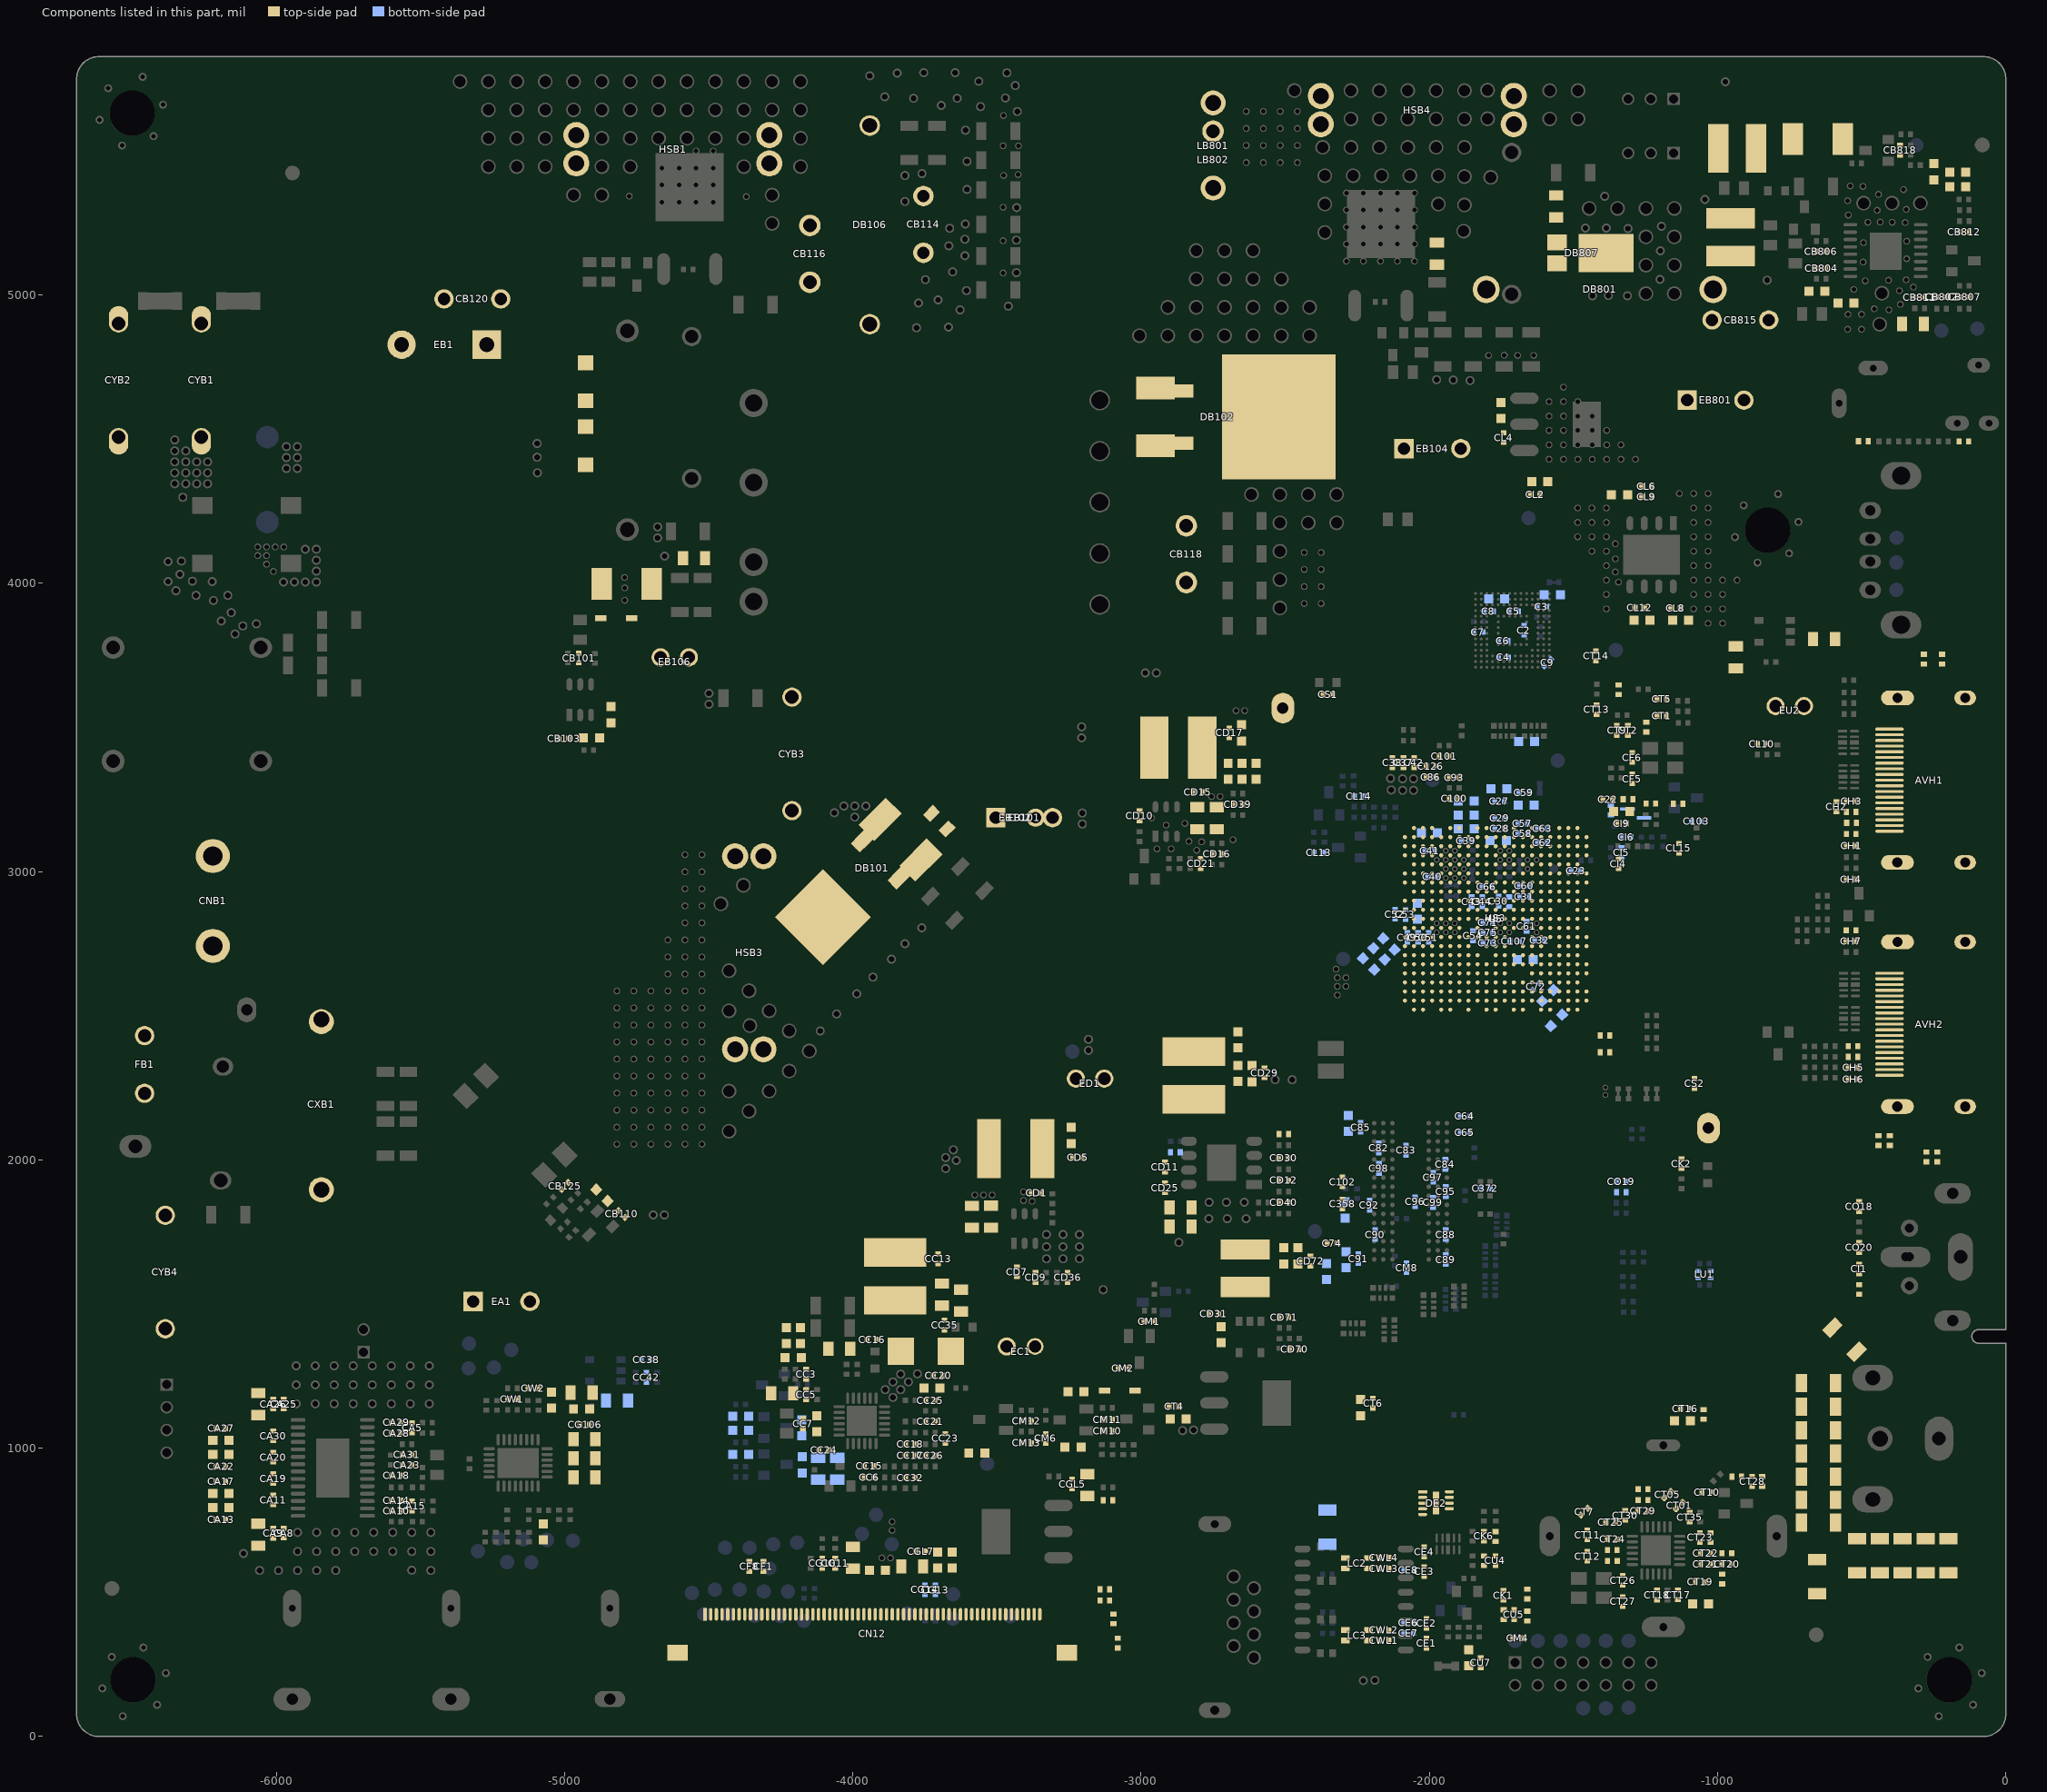
[diagram p0: the components of this part, seen from the top]
# Altium PCB MISC84395.PcbDoc (part 5 of 26)
Units mil, origin at the board's own origin, x right, y up, seen from the top; angles counter-clockwise.
Board outline 6692.91 x 5826.77 mil, 2 copper layers (TopLayer, BottomLayer), stack 61.855 mil thick; 951 components, 565 nets, 4374 pads, 1804 vias.
Unrouted connection lines stored in the file: 1.

## Footprints (in the part's own frame and the unit in brackets; to place one, negate y for a bottom-side part, rotate by r counter-clockwise, add the part's x,y. Pads: shape width x height; smd on the part's side, far side on the other; paste and mask are expansions set on the pad) (continued)
BGA406/0.8 [mm] "Mstar,MSD6A648WT-003J,16.12.17"
  round 0.36 smd: A2(-7.2,8) A3(-6.4,8) A5(-4.8,8) A6(-4,8) A8(-2.4,8) A9(-1.6,8) A11(0,8) A12(0.8,8) A14(2.4,8) A16(4,8) A17(4.8,8) A19(6.4,8) A20(7.2,8) AA2(-7.2,-8) AA3(-6.4,-8) AA4(-5.6,-8) AA6(-4,-8) AA7(-3.2,-8) AA9(-1.6,-8) AA10(-0.8,-8) AA12(0.8,-8) AA13(1.6,-8) AA15(3.2,-8) AA16(4,-8) AA18(5.6,-8) AA19(6.4,-8) AA20(7.2,-8) B1(-8,7.2) B2(-7.2,7.2) B3(-6.4,7.2) B4(-5.6,7.2) B5(-4.8,7.2) B6(-4,7.2) B7(-3.2,7.2) B8(-2.4,7.2) B9(-1.6,7.2) B10(-0.8,7.2) B11(0,7.2) B12(0.8,7.2) B13(1.6,7.2) B14(2.4,7.2) B15(3.2,7.2) B16(4,7.2) B17(4.8,7.2) B18(5.6,7.2) B19(6.4,7.2) B20(7.2,7.2) C1(-8,6.4) C2(-7.2,6.4) C3(-6.4,6.4) C4(-5.6,6.4) C5(-4.8,6.4) C6(-4,6.4) C7(-3.2,6.4) C8(-2.4,6.4) C9(-1.6,6.4) C10(-0.8,6.4) C11(0,6.4) C12(0.8,6.4) C13(1.6,6.4) C14(2.4,6.4) C15(3.2,6.4) C16(4,6.4) C17(4.8,6.4) C18(5.6,6.4) C19(6.4,6.4) C20(7.2,6.4) C21(8,6.4) D2(-7.2,5.6) D3(-6.4,5.6) D4(-5.6,5.6) D5(-4.8,5.6) D6(-4,5.6) D7(-3.2,5.6) D8(-2.4,5.6) D9(-1.6,5.6) D10(-0.8,5.6) D11(0,5.6) D12(0.8,5.6) D13(1.6,5.6) D14(2.4,5.6) D15(3.2,5.6) D16(4,5.6) D17(4.8,5.6) D18(5.6,5.6) D19(6.4,5.6) D20(7.2,5.6) D21(8,5.6) E1(-8,4.8) E2(-7.2,4.8) E3(-6.4,4.8) E4(-5.6,4.8) E5(-4.8,4.8) E6(-4,4.8) E7(-3.2,4.8) E10(-0.8,4.8) E11(0,4.8) E12(0.8,4.8) E13(1.6,4.8) E14(2.4,4.8) E15(3.2,4.8) E16(4,4.8) E17(4.8,4.8) E18(5.6,4.8) E19(6.4,4.8) E20(7.2,4.8) E21(8,4.8) F1(-8,4) F2(-7.2,4) F3(-6.4,4) F4(-5.6,4) F5(-4.8,4) F6(-4,4) F7(-3.2,4) F8(-2.4,4) F9(-1.6,4) F10(-0.8,4) F11(0,4) F12(0.8,4) F13(1.6,4) F14(2.4,4) F15(3.2,4) F16(4,4) F17(4.8,4) F18(5.6,4) F19(6.4,4) F20(7.2,4) F21(8,4) G2(-7.2,3.2) G3(-6.4,3.2) G4(-5.6,3.2) G5(-4.8,3.2) G6(-4,3.2) G7(-3.2,3.2) G8(-2.4,3.2) G9(-1.6,3.2) G10(-0.8,3.2) G11(0,3.2) G13(1.6,3.2) G14(2.4,3.2) G15(3.2,3.2) G16(4,3.2) G17(4.8,3.2) G18(5.6,3.2) G19(6.4,3.2) G20(7.2,3.2) G21(8,3.2) H1(-8,2.4) H2(-7.2,2.4) H3(-6.4,2.4) H4(-5.6,2.4) H6(-4,2.4) H7(-3.2,2.4) H8(-2.4,2.4) H10(-0.8,2.4) H11(0,2.4) H12(0.8,2.4) H14(2.4,2.4) H15(3.2,2.4) H16(4,2.4) H17(4.8,2.4) H18(5.6,2.4) H19(6.4,2.4) H20(7.2,2.4) H21(8,2.4) J1(-8,1.6) J2(-7.2,1.6) J3(-6.4,1.6) J4(-5.6,1.6) J5(-4.8,1.6) J6(-4,1.6) J7(-3.2,1.6) J10(-0.8,1.6) J11(0,1.6) J12(0.8,1.6) J13(1.6,1.6) J14(2.4,1.6) J15(3.2,1.6) J16(4,1.6) J17(4.8,1.6) J18(5.6,1.6) J19(6.4,1.6) J20(7.2,1.6) J21(8,1.6) K2(-7.2,0.8) K3(-6.4,0.8) K4(-5.6,0.8) K5(-4.8,0.8) K6(-4,0.8) K7(-3.2,0.8) K8(-2.4,0.8) K9(-1.6,0.8) K10(-0.8,0.8) K11(0,0.8) K13(1.6,0.8) K15(3.2,0.8) K16(4,0.8) K17(4.8,0.8) K18(5.6,0.8) K19(6.4,0.8) K20(7.2,0.8) K21(8,0.8) L1(-8,0) L2(-7.2,0) L3(-6.4,0) L4(-5.6,0) L5(-4.8,0) L6(-4,0) L7(-3.2,0) L8(-2.4,0) L9(-1.6,0) L10(-0.8,0) L11(0,0) L12(0.8,0) L13(1.6,0) L14(2.4,0) L15(3.2,0) L16(4,0) L17(4.8,0) L18(5.6,0) L19(6.4,0) L20(7.2,0) M1(-8,-0.8) M2(-7.2,-0.8) M5(-4.8,-0.8) M6(-4,-0.8) M7(-3.2,-0.8) M8(-2.4,-0.8) M9(-1.6,-0.8) M10(-0.8,-0.8) M11(0,-0.8) M12(0.8,-0.8) M13(1.6,-0.8) M14(2.4,-0.8) M15(3.2,-0.8) M16(4,-0.8) M17(4.8,-0.8) M18(5.6,-0.8) M19(6.4,-0.8) M20(7.2,-0.8) M21(8,-0.8) N1(-8,-1.6) N2(-7.2,-1.6) N3(-6.4,-1.6) N4(-5.6,-1.6) N5(-4.8,-1.6) N6(-4,-1.6) N7(-3.2,-1.6) N8(-2.4,-1.6) N9(-1.6,-1.6) N10(-0.8,-1.6) N11(0,-1.6) N12(0.8,-1.6) N13(1.6,-1.6) N14(2.4,-1.6) N15(3.2,-1.6) N16(4,-1.6) N17(4.8,-1.6) N18(5.6,-1.6) N19(6.4,-1.6) N20(7.2,-1.6) N21(8,-1.6) P2(-7.2,-2.4) P3(-6.4,-2.4) P4(-5.6,-2.4) P5(-4.8,-2.4) P6(-4,-2.4) P7(-3.2,-2.4) P8(-2.4,-2.4) P9(-1.6,-2.4) P10(-0.8,-2.4) P11(0,-2.4) P12(0.8,-2.4) P13(1.6,-2.4) P14(2.4,-2.4) P15(3.2,-2.4) P16(4,-2.4) P17(4.8,-2.4) P18(5.6,-2.4) P19(6.4,-2.4) P20(7.2,-2.4) R1(-8,-3.2) R2(-7.2,-3.2) R3(-6.4,-3.2) R4(-5.6,-3.2) R5(-4.8,-3.2) R6(-4,-3.2) R7(-3.2,-3.2) R8(-2.4,-3.2) R9(-1.6,-3.2) R10(-0.8,-3.2) R11(0,-3.2) R12(0.8,-3.2) R13(1.6,-3.2) R14(2.4,-3.2) R15(3.2,-3.2) R16(4,-3.2) R17(4.8,-3.2) R18(5.6,-3.2) R19(6.4,-3.2) R20(7.2,-3.2) R21(8,-3.2) T1(-8,-4) T2(-7.2,-4) T3(-6.4,-4) T4(-5.6,-4) T5(-4.8,-4) T6(-4,-4) T7(-3.2,-4) T8(-2.4,-4) T9(-1.6,-4) T10(-0.8,-4) T11(0,-4) T12(0.8,-4) T13(1.6,-4) T14(2.4,-4) T15(3.2,-4) T16(4,-4) T17(4.8,-4) T18(5.6,-4) T19(6.4,-4) T20(7.2,-4) T21(8,-4) U2(-7.2,-4.8) U3(-6.4,-4.8) U4(-5.6,-4.8) U5(-4.8,-4.8) U6(-4,-4.8) U7(-3.2,-4.8) U8(-2.4,-4.8) U9(-1.6,-4.8) U10(-0.8,-4.8) U11(0,-4.8) U12(0.8,-4.8) U13(1.6,-4.8) U14(2.4,-4.8) U15(3.2,-4.8) U16(4,-4.8) U17(4.8,-4.8) U18(5.6,-4.8) U19(6.4,-4.8) U20(7.2,-4.8) V1(-8,-5.6) V2(-7.2,-5.6) V3(-6.4,-5.6) V4(-5.6,-5.6) V5(-4.8,-5.6) V6(-4,-5.6) V7(-3.2,-5.6) V8(-2.4,-5.6) V9(-1.6,-5.6) V10(-0.8,-5.6) V11(0,-5.6) V12(0.8,-5.6) V13(1.6,-5.6) V14(2.4,-5.6) V15(3.2,-5.6) V16(4,-5.6) V17(4.8,-5.6) V18(5.6,-5.6) V19(6.4,-5.6) V20(7.2,-5.6) V21(8,-5.6) W1(-8,-6.4) W2(-7.2,-6.4) W3(-6.4,-6.4) W4(-5.6,-6.4) W5(-4.8,-6.4) W6(-4,-6.4) W7(-3.2,-6.4) W8(-2.4,-6.4) W9(-1.6,-6.4) W10(-0.8,-6.4) W11(0,-6.4) W12(0.8,-6.4) W13(1.6,-6.4) W14(2.4,-6.4) W15(3.2,-6.4) W16(4,-6.4) W17(4.8,-6.4) W18(5.6,-6.4) W19(6.4,-6.4) W20(7.2,-6.4) W21(8,-6.4) Y1(-8,-7.2) Y2(-7.2,-7.2) Y3(-6.4,-7.2) Y4(-5.6,-7.2) Y5(-4.8,-7.2) Y6(-4,-7.2) Y7(-3.2,-7.2) Y8(-2.4,-7.2) Y9(-1.6,-7.2) Y10(-0.8,-7.2) Y11(0,-7.2) Y12(0.8,-7.2) Y13(1.6,-7.2) Y14(2.4,-7.2) Y15(3.2,-7.2) Y16(4,-7.2) Y17(4.8,-7.2) Y18(5.6,-7.2) Y19(6.4,-7.2) Y20(7.2,-7.2) Y21(8,-7.2)
  round 0.36 smd mask+0.102: B21(8,7.2)
  silkscreen extent -9.62,-8.8 8.8,9.67, body extent -8.8,-8.8 8.8,8.8, height 1.6
C0402#1 [mm] "片式电容  2018.10.7 替换为兼容0201封装"
  rect 0.45x0.5 smd mask+0.051: 1(-0.425,0) 1(-0.425,0) 2(0.425,0) 2(0.425,0)
  silkscreen extent -0.88,-0.4 0.88,0.4
C0402#2 [mm] "片式电容  2018.10.7 替换为兼容0201封装"
  rrect50% 0.45x0.5 smd mask+0.051: 1(-0.425,0) 2(0.425,0)
  rect 0.3x0.3 smd mask+0.051: 1(-0.25,0) 2(0.25,0)
  rect 0.6x0.6 on Top Solder: 2(0,0)
  TopLayer pour cut-out: -0.318,0.302 -0.318,-0.303 0.306,-0.303 0.306,0.302
  silkscreen extent -0.88,-0.4 0.88,0.4, body extent -0.5,-0.25 0.5,0.25, height 0.5
C0603 [mm] "片式电容"
  rect 0.8x0.8 smd mask+0.076: 1(-0.706,0) 2(0.706,0)
  silkscreen extent -1.39,-0.55 1.39,0.55, body extent -0.8,-0.4 0.8,0.4, height 0.8
C0805 [mm] "片式电容"
  rect 0.9x1.25 smd mask+0.076: 1(-0.966,0) 2(0.966,0)
  silkscreen extent -1.73,-0.78 1.73,0.78, body extent -1,-0.62 1,0.63, height 1.25
C1206 [mm] "片式电容"
  rect 1x1.6 smd mask+0.076: 1(-1.5,-0.001) 2(1.5,0.001)
  silkscreen extent -2.39,-0.95 2.39,0.95, body extent -1.6,-0.8 1.6,0.8, height 1.3
CAP6.5*5-V-5-1 [mm] "TDK，CC45SL3DD680JYSNA，外K型引脚，AI，0713_2018"
  round 2.1 on Top Overlay: 0(-2.5,0) 0(2.5,0)
  round 1.9 hole 1.2 mask+0.051: 1(-2.5,0) 2(2.5,0)
  BottomLayer lines w0.6: -2.19,0.39 -4.056,1.556 ; 2.89,0.31 4.056,-1.556 ; -2.5,0 -4.056,1.556 ; 2.5,0 4.056,-1.556 ; -2.89,-0.31 -4.056,1.556 ; 2.19,-0.39 4.056,-1.556
  silkscreen extent -5.5,-2.5 5.5,2.5
CAP7.5*2.5-V-5 [mm] "同皓电子"
  round 1.7 hole 1.1: 1(-2.5,0) 2(2.5,0)
  round 1.9 on Top Overlay: 43(2.5,0) 44(-2.5,0)
  BottomLayer lines w0.6: -2.89,-0.31 -2.92,-0.262 ; -2.5,0 -2.729,0.229 -4.056,1.556 ; -2.19,0.39 -2.238,0.42 ; 2.19,-0.39 2.238,-0.42 2.5,-0.584 4.056,-1.556 ; 2.5,0 4.056,-1.556 ; 2.89,0.31 2.92,0.262 4.056,-1.556 ; -4.056,1.556 -2.238,0.42 ; -4.056,1.556 -3.035,-0.078 -2.92,-0.262 ; -2.92,-0.262 -2.92,-0.262 ; -2.92,-0.262 -2.92,-0.262 ; -2.238,0.42 -2.238,0.42 ; -2.238,0.42 -2.238,0.42
  silkscreen extent -3.75,-1.25 3.75,1.25, body extent -3.75,-1.25 3.75,1.25, height 8.5
CAP8*2.5-V-5 [mm] "C242G472J20A201(编带/法拉)"
  round 1.8 hole 1.1: 1(-2.5,0) 2(2.5,0)
  round 2 on Top Overlay: 1(-2.5,0) 1(2.5,0)
  BottomLayer lines w0.6: 2.15,-0.456 4.056,-1.556 ; -2.956,-0.35 -4.056,1.556 ; 2.5,0 4.056,-1.556 ; -2.5,0 -4.056,1.556 ; 2.956,0.35 3.157,0 4.056,-1.556 ; -2.15,0.456 -4.056,1.556
  silkscreen extent -4,-1.25 4,1.25
CAP8.5*5-V-5 [mm] "TDK，CC45SL3AD221JYSNA，外K型引脚，AI，0713_2018"
  round 2.1 on Top Overlay: 0(-2.5,0) 0(2.5,0)
  round 1.9 hole 1.2 mask+0.051: 1(-2.5,0) 2(2.5,0)
  BottomLayer lines w0.6: 2.19,-0.39 4.056,-1.556 ; -2.89,-0.31 -4.056,1.556 ; 2.5,0 4.056,-1.556 ; -2.5,0 -4.056,1.556 ; 2.89,0.31 4.056,-1.556 ; -2.19,0.39 -4.056,1.556
  silkscreen extent -5.5,-2.5 5.5,2.5
CAP10*4.5-V-5 [mm] "YU102472M090DAND5H，陶瓷电容，17.12.22"
  round 1.7 hole 1.1: 1(-2.5,0) 2(2.5,0)
  round 1.9 on Top Overlay: 41(2.5,0) 42(-2.5,0)
  BottomLayer lines w0.6: -2.89,-0.31 -2.92,-0.262 ; -2.5,0 -4.056,1.556 ; -2.19,0.39 -2.238,0.42 ; 2.19,-0.39 2.238,-0.42 ; 2.5,0 4.056,-1.556 ; 2.89,0.31 2.92,0.262 ; -4.056,1.556 -2.92,-0.262 ; -4.056,1.556 -2.238,0.42 ; -2.92,-0.262 -2.92,-0.262 ; -2.92,-0.262 -2.92,-0.262 ; -2.238,0.42 -2.238,0.42 ; -2.238,0.42 -2.238,0.42 ; 2.238,-0.42 2.238,-0.42 ; 2.238,-0.42 2.238,-0.42 ; 2.238,-0.42 2.439,-0.545 4.056,-1.556 ; 2.92,0.262 2.92,0.262 4.056,-1.556 ; 2.92,0.262 2.92,0.262
  silkscreen extent -5.55,-2.25 5.55,2.25
CAP13*5-V-10-1#1 [mm] "Walsin;YU1AH471M060DAMD0H;160718（18.03.15  更新孔径）"
  oval 2.35x1.7 hole 1.2 copper offset -0.375,0: 1(-5,0)
  oval 2.35x1.7 hole 1.2 copper offset 0.375,0: 2(5,0)
  oval 2.55x1.9 on Top Overlay: 61(-5,0) 61(5,0)
  silkscreen extent -5.71,-3 5.81,3
CAP13*5-V-10-1#2 [mm] "Walsin;YU1AH471M060DAMD0H;160718（18.03.15  更新孔径）"
  round 1.7 hole 1.2: 1(-5,0) 2(5,0)
  round 1.9 on Top Overlay: 61(-5,0) 61(5,0)
  silkscreen extent -5.71,-3 5.81,3
CAP18*8.5-V-15 [mm] "PX334K3ID49H200D9R(凯励)(18.01.12更新孔径）(18.07.18 更新丝印框，加了公差）"
  round 2.2 hole 1.4: 1(-7.5,0)
  round 2.2 hole 1.4 copper offset -0.2,0: 2(7.5,0)
  round 2.4 on Top Overlay: 77(7.5,0) 78(-7.5,0)
  silkscreen extent -9.25,-4.45 9.25,4.45
CAUTION [mil]
  silkscreen extent -400,-146 486,161
COLD [mil]
CON2-H7.92 [mm] "因物料底部露金属，20170630增加1.8mm安规禁布"
  round 3 / inner round 3 / far side round 4.4 hole 1.7: 1(0,3.96) 3(0,-3.96)
  round 3.2 on Top Overlay: 109(0,3.96) 110(0,-3.96)
  silkscreen extent -12,-6.52 4.27,8.46, body extent -11.46,-6.04 0.56,5.86, height 8.49
"Conformal Coating" [mm] "三防漆虚线框"
  round 0.3 on Mech2: 0(0,0)
CQC [mil]
D1-H-17.5 [mm] "FR107 二极管与FR207 共用封装"
  round 2 on Top Overlay: 0(-8.75,0) 1(8.75,0)
  round 1.8 hole 1.3: A(-8.75,0) K(8.75,0)
  BottomLayer lines w0.6: -8.675,0.569 -6.55,0 ; 8.675,0.569 6.55,0 ; -8.75,0 -6.55,0 ; 8.75,0 6.55,0 ; -8.675,-0.569 -6.55,0 ; 8.675,-0.569 6.55,0
  silkscreen extent -7.8,-1.65 7.7,1.65, body extent -9.13,-1.49 9.13,1.5, height 3.15
D2PAK3#1 [mm] "伟达电子；SFS1006G;增加TO-252兼容；160309"
  oval 2.794x1.143 smd: 1(5.542,-2.2) 3(5.542,2.4)
  rect 2.794x1.143 smd: 1(5.544,-2.2) 3(5.544,2.4)
  rect 3.4x2 smd paste-5 mask-5: 1(7.494,-2.44) 3(7.494,2.64)
  rect 6x6 smd paste-10 mask-11: 2(-2.159,0.1)
  TopLayer pour cut-out: 3.373,2.4 6.497,2.4 6.497,-2.245 6.438,-2.54 6.271,-2.791 6.02,-2.958 5.725,-3.017 5.725,-3.017 5.725,-2.199 4.141,-2.199 4.141,-3.024 3.847,-2.966 3.598,-2.799 3.432,-2.55 3.373,-2.256 3.373,-2.256
  silkscreen extent -9.13,-5.69 4.84,5.89, body extent -6.91,-5.15 8.79,5.35, height 4.7
D2PAK3#2 [mm] "伟达电子；SFS1006G;增加TO-252兼容；160309"
  oval 2.794x1.143 smd: 1(5.542,-2.2) 3(5.542,2.4)
  rect 2.794x1.143 smd: 1(5.544,-2.2) 3(5.544,2.4)
  rect 3.4x2 smd paste-5 mask-5: 1(7.494,-2.44) 3(7.494,2.64)
  rect 10x11 smd paste-11 mask-11: 2(-3.356,0.1)
  rect 6x6 smd paste-10 mask-11: 2(-2.158,0.1)
  TopLayer pour cut-out: 3.373,2.4 6.497,2.4 6.497,-2.245 6.438,-2.54 6.271,-2.791 6.02,-2.958 5.725,-3.017 5.725,-3.017 5.725,-2.199 4.141,-2.199 4.141,-3.024 3.847,-2.966 3.598,-2.799 3.432,-2.55 3.373,-2.256 3.373,-2.256
  silkscreen extent -9.13,-5.69 4.84,5.89, body extent -6.91,-5.15 8.79,5.35, height 4.7
D3-H-20 [mm] "肖特基二极管"
  round 2.6 on Top Overlay: 0(10,0) 1(-10,0)
  round 2.4 hole 1.6: A(-10,0) K(10,0)
  silkscreen extent -13,-2.6 13,2.6, body extent -12.62,-2.69 12.63,2.69, height 11.81
DFN10/0.5-2 [mm] "晶焱；AZ3133-04F;15.09.18"
  rect 0.8x0.28 smd mask+0.102: 1(-1.175,1)
  oval 0.8x0.28 smd mask+0.102: 2(-1.175,0.5) 3(-1.175,0) 4(-1.175,-0.5) 5(-1.175,-1) 7(1.175,-0.5) 8(1.175,0) 9(1.175,0.5) 10(1.175,1)
  oval 0.8x0.28 on Top Overlay mask+0.102: 6(1.175,-1)
  rect 0.584x0.85 on Top Solder paste-16 mask-16: EPAD(0,-0.575) EPAD(0,0.575)
  rect 0.584x2 smd paste-5 mask-5: EPAD(0,0)
  rect 0.584x0.85 on Top Paste paste-16 mask-16: EPAD(0,-0.575) EPAD(0,0.575)
  silkscreen extent -2.52,-1.33 1.28,1.4, body extent -1.28,-1.28 1.28,1.28, height 0.6
DIODE-S0402 [mm] "DVD上使用的ESD"
  rect 0.45x0.55 smd mask+0.051: A(-0.425,0) K(0.425,0)
  silkscreen extent -0.8,-0.43 0.91,0.43, body extent -0.5,-0.25 0.5,0.25, height 0.5
DIODE-S-1 [mm] "SK34(18.09.07 去除0805电阻兼容）"
  rect 2.33x2.4 smd: A(-2.21,0) K(2.21,0)
  silkscreen extent -3.8,-1.4 4.04,1.4, body extent -2.63,-1.12 2.37,1.12, height 2
DIODE-S-2 [mm] "1N5819-SMA;170509去除兼容,20180607减少内距0.4mm以兼容SMAF"
  rect 1.8x2.8 smd: A(-2.2,0) K(2.2,0)
  silkscreen extent -3.5,-1.6 3.7,1.61, body extent -2.6,-1.4 2.6,1.4, height 1.91
DIODE-S-12 [mm] "Formosa MS ;BAV19WS THRU BAV21WS/PMEG2010BEA(高度为1.1mm)"
  rect 1x0.55 smd: A(1.35,0) K(-1.35,0)
  silkscreen extent -0.9,-0.67 0.9,0.67, body extent -1.35,-0.63 1.35,0.63, height 1
DIODE-S-13 [mm] "DIODES;SBR10U45SP5"
  rect 1.4x1.75 smd: 1(0.92,-2.925) 3(-0.92,-2.925)
  rect 3.36x4.86 smd: 2(0,1.4)
  silkscreen extent -2.02,-2.73 2.02,2.73, body extent -2.02,-3.3 2.02,3.3, height 1.15
DIODE-S-14 [mm] "ROHM;FSL14"
  rect 1.3x1.35 smd: A(1.675,0) K(-1.675,0)
  silkscreen extent -1.55,-1 1.55,1, body extent -1.95,-1 1.95,1, height 1.08
"DOLBY PLUS-SILK" [mil]
  silkscreen extent -16,-177 1441,197
EC(5*11)-V-2.5#1 [mm] "机插2.5间距"
  round 1.8 on Top Overlay: 0(-1.25,0) 0(1.25,0)
  round 0.5 on Keep-Out: 0(0,-0.787)
  round 1.6 hole 1.1: 1(-1.25,0) 2(1.25,0)
  BottomLayer lines w0.6: -1.64,-0.31 -1.67,-0.262 ; -1.25,0 -2.806,1.556 ; -0.94,0.39 -0.988,0.42 ; 0.94,-0.39 0.988,-0.42 ; 1.25,0 1.453,-0.203 2.806,-1.556 ; 1.64,0.31 1.67,0.262 1.67,0.262 ; -2.806,1.556 -1.25,0.584 -0.988,0.42 ; -2.806,1.556 -1.67,-0.262 ; -1.67,-0.262 -1.67,-0.262 ; -1.67,-0.262 -1.67,-0.262 ; -0.988,0.42 -0.988,0.42 ; -0.988,0.42 -0.988,0.42 ; 0.988,-0.42 0.988,-0.42 ; 0.988,-0.42 2.806,-1.556 ; 0.988,-0.42 0.988,-0.42 ; 1.67,0.262 1.67,0.262 ; 1.67,0.262 1.765,0.109 2.806,-1.556
  silkscreen extent -2.75,-2.75 3,2.75, body extent -2.48,-2.52 2.5,2.47, height 12.5
EC(5*11)-V-2.5#2 [mm] "机插2.5间距"
  round 1.8 on Top Overlay: 0(-1.25,0) 0(1.25,0)
  round 0.5 on Keep-Out: 0(0,-0.787)
  round 1.6 hole 1.1: 1(-1.25,0) 2(1.25,0)
  BottomLayer lines w0.6: -1.64,-0.31 -1.67,-0.262 -2.806,1.556 ; -1.25,0 -2.806,1.556 ; -0.94,0.39 -0.988,0.42 -2.806,1.556 ; 0.94,-0.39 0.988,-0.42 2.806,-1.556 ; 1.25,0 2.806,-1.556 ; 1.64,0.31 1.67,0.262 2.806,-1.556
  silkscreen extent -2.75,-2.75 3,2.75, body extent -2.48,-2.52 2.5,2.47, height 12.5
EC(6.3*11)-V-2.5#1 [mm] "机插2.5间距"
  round 0.5 on Keep-Out: 0(0,-0.889)
  round 1.6 hole 1.1: 1(-1.25,0)
  round 1.473 / inner round 1.6 / far side round 1.6 hole 1.1: 2(1.25,0)
  round 1.8 on Top Overlay: 5(1.25,0) 6(-1.25,0)
  BottomLayer lines w0.6: -1.665,-0.275 -2.664,1.685 ; -1.25,0 -2.664,1.685 ; -0.907,0.361 -2.664,1.685 ; 0.907,-0.361 0.952,-0.395 2.664,-1.685 ; 1.25,0 2.664,-1.685 ; 1.665,0.275 1.691,0.225 2.664,-1.685
  silkscreen extent -3.17,-3.17 3.51,3.17, body extent -3,-3 2.98,2.99, height 12.5
EC(6.3*11)-V-2.5#2 [mm] "机插2.5间距"
  round 0.5 on Keep-Out: 0(0,-0.889)
  round 1.6 hole 1.1: 1(-1.25,0) 2(1.25,0)
  round 1.8 on Top Overlay: 5(1.25,0) 6(-1.25,0)
  BottomLayer lines w0.6: -1.665,-0.275 -2.664,1.685 ; -1.25,0 -1.569,0.38 -2.664,1.685 ; -0.907,0.361 -0.952,0.395 -1.256,0.624 -2.664,1.685 ; 0.907,-0.361 0.952,-0.395 2.664,-1.685 ; 1.25,0 2.664,-1.685 ; 1.665,0.275 1.691,0.225 2.664,-1.685
  silkscreen extent -3.17,-3.17 3.51,3.17, body extent -3,-3 2.98,2.99, height 12.5
EC(8*11)-V-3.5 [mm]
  rect 1.6x1.6 hole 1: 1(-1.75,0)
  rect 1.8x1.8 on Top Overlay: 1(-1.75,0)
  round 1.8 on Top Overlay: 1(1.75,0)
  round 1.6 hole 1: 2(1.75,0)
  silkscreen extent -4.25,-4.25 4.45,4.25, body extent -3.98,-3.98 4.01,4.01, height 12.51
EC(10*12)-V-5 [mm] "机插5间距"
  rect 1.9x1.9 on Top Overlay: 0(-2.5,0)
  round 0.5 on Keep-Out: 0(-0.75,0)
  round 1.9 on Top Overlay: 0(2.5,0)
  rect 1.7x1.7 hole 1.1: 1(-2.5,0)
  round 1.7 hole 1.1: 2(2.5,0)
  BottomLayer lines w0.6: -2.89,-0.31 -2.92,-0.262 ; -2.5,0 -4.056,1.556 ; -2.19,0.39 -2.238,0.42 ; 2.19,-0.39 2.238,-0.42 4.056,-1.556 ; 2.5,0 4.056,-1.556 ; 2.89,0.31 2.92,0.262 4.056,-1.556 ; -4.056,1.556 -2.92,-0.262 ; -4.056,1.556 -2.238,0.42 ; -2.92,-0.262 -2.92,-0.262 ; -2.238,0.42 -2.238,0.42
  silkscreen extent -5.25,-5.25 5.57,5.25, body extent -4.98,-4.99 5.01,4.99, height 12.01
EC(10*12.5)-V-5#1 [mm] "机插5间距"
  round 0.5 on Keep-Out: 0(-0.75,0)
  rect 1.7x1.7 hole 1.1: 1(-2.5,0)
  rect 1.9x1.9 on Top Overlay: 1(-2.5,0)
  round 1.9 on Top Overlay: 1(2.5,0)
  round 1.7 hole 1.1: 2(2.5,0)
  BottomLayer lines w0.6: -2.89,-0.31 -2.92,-0.262 -3.634,0.881 -4.056,1.556 ; -2.5,0 -3.381,0.881 -4.056,1.556 ; -2.19,0.39 -2.238,0.42 -4.056,1.556 ; 2.19,-0.39 2.238,-0.42 2.5,-0.584 4.056,-1.556 ; 2.5,0 4.056,-1.556 ; 2.89,0.31 2.92,0.262 ; 2.92,0.262 3.084,0 4.056,-1.556
  silkscreen extent -5.2,-5.21 5.57,5.21, body extent -4.98,-4.99 5.01,4.99, height 14.01
EC(10*12.5)-V-5#2 [mm] "机插5间距"
  round 0.5 on Keep-Out: 0(-0.75,0)
  rect 1.7x1.7 hole 1.1: 1(-2.5,0)
  rect 1.9x1.9 on Top Overlay: 1(-2.5,0)
  round 1.9 on Top Overlay: 1(2.5,0)
  round 1.7 hole 1.1: 2(2.5,0)
  BottomLayer lines w0.6: -2.89,-0.31 -2.92,-0.262 ; -2.5,0 -4.056,1.556 ; -2.19,0.39 -2.238,0.42 ; 2.19,-0.39 2.238,-0.42 ; 2.5,0 4.056,-1.556 ; 2.89,0.31 2.92,0.262 2.92,0.262 ; -4.056,1.556 -2.5,0.584 -2.238,0.42 ; -4.056,1.556 -2.92,-0.262 ; -2.92,-0.262 -2.92,-0.262 ; -2.92,-0.262 -2.92,-0.262 ; -2.238,0.42 -2.238,0.42 ; -2.238,0.42 -2.238,0.42 ; 2.238,-0.42 2.238,-0.42 ; 2.238,-0.42 2.238,-0.42 ; 2.238,-0.42 2.385,-0.512 2.5,-0.584 4.056,-1.556 ; 2.92,0.262 2.92,0.262 ; 2.92,0.262 4.056,-1.556
  silkscreen extent -5.2,-5.21 5.57,5.21, body extent -4.98,-4.99 5.01,4.99, height 14.01
EC(10*12.5)-V-5#3 [mm] "机插5间距"
  round 0.5 on Keep-Out: 0(-0.75,0)
  rect 1.7x1.7 hole 1.1: 1(-2.5,0)
  rect 1.9x1.9 on Top Overlay: 1(-2.5,0)
  round 1.9 on Top Overlay: 1(2.5,0)
  round 1.7 hole 1.1: 2(2.5,0)
  BottomLayer lines w0.6: -2.89,-0.31 -2.92,-0.262 ; -2.5,0 -3.378,0.878 -4.056,1.556 ; -2.19,0.39 -2.238,0.42 ; 2.19,-0.39 2.238,-0.42 ; 2.5,0 2.906,-0.406 4.056,-1.556 ; 2.89,0.31 2.906,0.284 2.92,0.262 ; -4.056,1.556 -2.92,-0.262 ; -4.056,1.556 -3.378,1.132 -2.4,0.521 -2.238,0.42 ; -2.92,-0.262 -2.92,-0.262 ; -2.92,-0.262 -2.92,-0.262 ; -2.238,0.42 -2.238,0.42 ; -2.238,0.42 -2.238,0.42 ; 2.238,-0.42 2.238,-0.42 ; 2.238,-0.42 2.5,-0.584 2.906,-0.838 4.056,-1.556 ; 2.92,0.262 2.92,0.262 ; 2.92,0.262 4.056,-1.556
  silkscreen extent -5.2,-5.21 5.57,5.21, body extent -4.98,-4.99 5.01,4.99, height 14.01
EC(18*41)-H-7.5-1 [mm] "SAMXON  (18*40)，开槽"
  round 2.7 on Top Overlay: 1(-3.75,2.5)
  rect 2.5x2.5 hole 1.3: 1(3.75,2.5)
  rect 2.7x2.7 on Top Overlay: 1(3.75,2.5)
  round 2.5 hole 1.3: 2(-3.75,2.5)
  KeepOutLayer lines w0.127: -6.75,-46.5 6.75,-46.5 6.75,-2 -6.75,-2 -6.75,-46.5
  silkscreen extent -9.25,-46 9.25,2.5
EVA(7*7*3) [mil] "7*7*3"
  silkscreen extent -177,-177 177,177
FFC60H/0.5S-13 [mm] "FOOSUNG,CAAAR060A,前掀盖，掀盖最大高度4.1mm，19.04.24"
  rect 0.3x1.1 smd mask+0.076: 1(-14.75,1.697)
  oval 0.3x1.1 smd mask+0.076: 2(-14.25,1.697) 3(-13.75,1.697) 4(-13.25,1.697) 5(-12.75,1.697) 6(-12.25,1.697) 7(-11.75,1.697) 8(-11.25,1.697) 9(-10.75,1.697) 10(-10.25,1.697) 11(-9.75,1.697) 12(-9.25,1.697) 13(-8.75,1.697) 14(-8.25,1.697) 15(-7.75,1.697) 16(-7.25,1.697) 17(-6.75,1.697) 18(-6.25,1.697) 19(-5.75,1.697) 20(-5.25,1.697) 21(-4.75,1.697) 22(-4.25,1.697) 23(-3.75,1.697) 24(-3.25,1.697) 25(-2.75,1.697) 26(-2.25,1.697) 27(-1.75,1.697) 28(-1.25,1.697) 29(-0.75,1.697) 30(-0.25,1.697) 31(0.25,1.697) 32(0.75,1.697) 33(1.25,1.697) 34(1.75,1.697) 35(2.25,1.697) 36(2.75,1.697) 37(3.25,1.697) 38(3.75,1.697) 39(4.25,1.697) 40(4.75,1.697) 41(5.25,1.697) 42(5.75,1.697) 43(6.25,1.697) 44(6.75,1.697) 45(7.25,1.697) 46(7.75,1.697) 47(8.25,1.697) 48(8.75,1.697) 49(9.25,1.697) 50(9.75,1.697) 51(10.25,1.697) 52(10.75,1.697) 53(11.25,1.697) 54(11.75,1.697) 55(12.25,1.697) 56(12.75,1.697) 57(13.25,1.697) 58(13.75,1.697) 59(14.25,1.697) 60(14.75,1.697)
  rect 1.8x1.4 smd mask+0.076: 61(-17.152,-1.703) 62(17.152,-1.703)
  TopLayer region: 16.565,0.446 16.296,0.446 16.296,-1.18 16.565,-1.18
  TopLayer region: -16.565,-1.18 -16.296,-1.18 -16.296,0.446 -16.565,0.446
  silkscreen extent -17.57,-3.55 17.58,3.3
Fixed [mm] "麦拉片塑胶固定柱(4.50×6.49mm-尼龙-白色)"
  round 2.5 on Keep-Out: 0(0,0)
  silkscreen extent -1.9,-1.9 1.9,1.9
"FUSE8.5*4-V-5(T3.15AL 250V~)" [mm] "SMT1315AP/2010T1A250VA1(编带/华德)"
  round 1.7 hole 1.15: 1(2.54,0) 2(-2.54,0)
  round 1.9 on Top Overlay: 4(2.54,0) 5(-2.54,0)
  BottomLayer lines w1: -2.312,0.271 -2.338,0.289 -3.977,1.437 ; 2.811,0.228 2.829,0.202 3.275,-0.434 3.977,-1.437 ; -2.54,0 -3.977,1.437 ; 2.54,0 3.124,-0.584 3.977,-1.437 ; -2.811,-0.228 -2.829,-0.202 -2.971,0 -3.977,1.437 ; 2.312,-0.271 2.338,-0.289 3.977,-1.437
  silkscreen extent -4.3,-2.1 4.3,2.1, body extent -4.3,-2.1 4.3,2.1, height 8.5
GND [mm] "导通线"
  rect 0.66x0.3 smd paste-0.45 mask-0.45: JP_1K(-0.32,0) JP_2K(0.32,0)
HDMI-HS-1 [mm] "浙江和丰   HHF-14B000-2SA。17.09.25更新钢网;171107更新焊盘露铜位置(18.04.19 更新大脚孔径）"
  rect 2.2x3.8 on Top Paste: 0(-7.75,4.18) 0(7.753,4.183)
  rect 2.2x6 on Top Paste: 0(-7.75,9.355) 0(7.75,9.355)
  oval 0.26x2.5 smd: 1(4.5,11.258) 2(4,11.258) 3(3.5,11.258) 4(3,11.258) 5(2.5,11.258) 6(2,11.258) 7(1.5,11.258) 8(1,11.258) 9(0.5,11.258) 10(0,11.258) 11(-0.5,11.258) 12(-1,11.258) 13(-1.5,11.258) 14(-2,11.258) 15(-2.5,11.258) 16(-3,11.258) 17(-3.5,11.258) 18(-4,11.258) 19(-4.5,11.258)
  oval 1.3x2.9 hole 0.9 slot 2.5 at 90 deg mask+0.076: 20(-7.25,10.565) 22(7.25,10.55)
  oval 1.3x1.9 hole 0.9 slot 1.5 at 90 deg mask+0.076: 21(-7.25,4.59) 23(7.25,4.59)
  silkscreen extent -7.5,2 7.5,12.19, body extent -10.25,-57.68 10.25,12.17, height 8.42
"Heat-Shrinkable Tube" [mm] "收缩前壁厚0.3+-0.05，收缩后壁厚0.6+-0.1"
  round 0.3 on Mech2: 0(0,0)
"High Voltage" [mil]
  silkscreen extent -21,-60 17,50
HOT [mil]
HS149-YZ [mm] "17.5×14.5×0.5-本色-Cu-LHD, 18.05.17  取代HS038的验证封装"
  round 2.3 hole 1.4: 1(-8.5,1.25) 2(-8.5,-1.25) 3(8.5,-1.25) 4(8.5,1.25)
  BottomLayer region: 7.983,-1.016 8.999,-1.016 8.999,1.016 7.983,1.016
  BottomLayer region: -9.017,-1.016 -8.001,-1.016 -8.001,1.016 -9.017,1.016
  silkscreen extent -8.5,-2.5 8.5,2.5
HS(40*40*2.3)-1 [mm] "Asink;40*40*2.3(散热片本体2.3mm);20170420,实物铣平铆钉"
  oval 2.7x2 hole 1 slot 1.7 at 0 deg: 1(-18.5,-18.75) 2(18.5,18.75)
  oval 2.9x2.2 on Top Overlay: 2(-18.5,-18.75) 2(18.5,18.75)
  silkscreen extent -20.27,-20.27 20.27,20.27, body extent -20.04,-20.02 20.09,20.02, height 2.5
L0402 [mm] "电感"
  rect 0.45x0.55 smd mask+0.076: 1(-0.425,0) 2(0.425,0)
  silkscreen extent -0.8,-0.42 0.8,0.43, body extent -0.5,-0.25 0.5,0.25, height 0.5
L0603 [mil] "片式磁珠、电感、ESD"
  rect 32x31.5 smd mask+3: 1(-27.81,0) 2(27.81,0)
  silkscreen extent -50,-22 50,22, body extent -31,-16 31,16, height 31
L(4.5*3.5)-S [mm] "SMD4532-6R8M-023"
  rect 1.8x4.3 smd: 1(-1.65,0) 2(1.65,0)
  TopLayer pour cut-out: -0.76,2.15 0.796,2.15 0.796,2.141 0.796,-2.149 -0.756,-2.149 -0.756,-2.15
  silkscreen extent -2.83,-2.44 3.3,2.44
L(5.8*4.5)-S [mm] "APC52A45M4R7\电感\Cailank;170317更新阻焊兼容L(4*3.0)-S"
  rect 2.5x5.5 smd paste-5.5: 1(2.105,0) 2(-2.105,0)
  TopLayer pour cut-out: -0.849,2.746 -0.845,2.75 0.861,2.75 0.861,-2.749 0.861,-2.753 0.859,-2.753 -0.862,-2.753
  silkscreen extent -1.5,-2.9 3.88,2.9, body extent -3.06,-2.65 3.08,2.74, height 4.8
L(6.0*4.5)-S [mm] "SWPA6045S4R7MT(Sunlord) :功率电感;161103更新焊盘大小"
  rect 2.1x5.2 smd paste-6: 1(-2.35,0) 2(2.35,0)
  TopLayer pour cut-out: -1.282,2.552 1.294,2.543 1.297,-2.547 -1.311,-2.549
  silkscreen extent -3.16,-3.15 3.9,3.15, body extent -3,-3 3,3, height 4.5
L(13.5*15.5)-V-5 [mm] "深圳秀益达；SA-A048-036-A SPK1214RBL-680K；14.11.19"
  round 1.9 hole 1.2 mask+0.076: 1(-2.5,0) 2(2.5,0)
  round 2.1 on Top Overlay mask+0.076: 3(-2.5,0) 4(2.5,0)
  silkscreen extent -6.75,-6.75 6.75,6.75, body extent -6.72,-6.73 6.72,6.75, height 15.5
L/LC2/15*14.5-V7.5 [mm] "SYDR1212-L003-YMX"
  round 2.2 hole 1.4: 1(-3.75,0) 2(3.75,0)
  round 2.4 on Top Overlay: 1(-3.75,0) 1(3.75,0)
  silkscreen extent -7.25,-7.25 7.25,7.25
L/LC4/1.25*1.0 [mil] "共模电感：DLP11S/R/T Series(muRata);S高度:0.92;R高度:0.6;T高度:0.35"
  rect 14x20 smd: 1(-11.81,-21.65) 2(-11.81,21.65) 3(11.81,21.65) 4(11.81,-21.65)
  silkscreen extent -28,-39 28,39, body extent -22,-27 22,27, height 36
L/LC4/2*1.2-S [mm] "台庆,WCM2012F2SF-801-N,17.09.21"
  rect 0.76x0.5 smd: 1(1.008,0.458) 2(-1.01,0.46) 3(-1.01,-0.46) 4(1.008,-0.462)
  silkscreen extent -1.1,-0.68 1.56,1.36